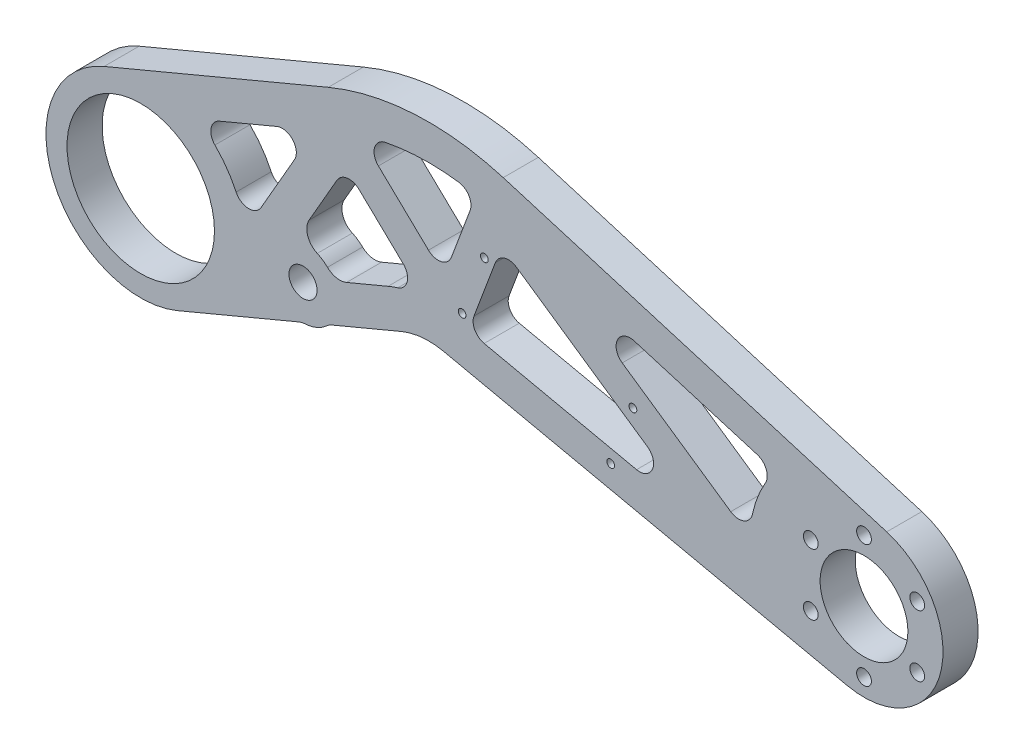
from build123d import *

# Parameters (mm, degrees)
SKETCH_1_R          = 21
SKETCH_1_R_2        = 12.5
EXTRUDE_1_DEPTH     = 10
EXTRUDE_3_DEPTH     = 10
CUT_EXTRUDE_1_DEPTH = 143.471558445
CUT_EXTRUDE_2_DEPTH = 143.471558445
FILLET_1_R          = 4
SKETCH_4_R          = 2.1
CUT_EXTRUDE_3_DEPTH = 143.471558445
SKETCH_5_R          = 4
CUT_EXTRUDE_4_DEPTH = 10
SKETCH_6_R          = 10
SKETCH_6_R_2        = 4
EXTRUDE_4_DEPTH     = 10
FILLET_2_R          = 5
SKETCH_7_R          = 1.1
CUT_EXTRUDE_5_DEPTH = 10


with BuildPart() as part:
    # 草图1 → 凸台-拉伸1 (new body)
    with BuildSketch(Plane.XY):
        with BuildLine():
            ThreePointArc((-102.410194175, 26.993557177), (-130, 0), (-102.410194175, -26.993557177))
            Line((-102.410194175, -26.993557177), (103.491504854, -22.494630981))
            ThreePointArc((103.491504854, -22.494630981), (125.5, 0), (103.491504854, 22.494630981))
            Line((103.491504854, 22.494630981), (-102.410194175, 26.993557177))
        make_face()
        with Locations((-103, 0)):
            Circle(SKETCH_1_R, mode=Mode.SUBTRACT)
        with Locations((103, 0)):
            Circle(SKETCH_1_R_2, mode=Mode.SUBTRACT)
    extrude(amount=EXTRUDE_1_DEPTH)

    # 草图2 → 凸台-拉伸3 (add)
    with BuildSketch(Plane(origin=(0, 0, 0), x_dir=(-1, 0, 0), z_dir=(0, 0, -1))):
        with BuildLine():
            Line((-103.491504854, 22.494630981), (-40.939702548, 23.861379985))
            ThreePointArc((-40.939702548, 23.861379985), (-23.289176704, 42.694903268), (-0.239881629, 54.312676651))
            Line((-0.239881629, 54.312676651), (-109.464232513, 21.551419861))
            ThreePointArc((-109.464232513, 21.551419861), (-106.509698333, 22.224581382), (-103.491504854, 22.494630981))
        make_face()
        with BuildLine():
            ThreePointArc((-0.239881629, 54.312676651), (-23.289176704, 42.694903268), (-40.939702548, 23.861379985))
            Line((-40.939702548, 23.861379985), (81.117648154, 26.528317728))
            ThreePointArc((81.117648154, 26.528317728), (67.102789284, 41.29360316), (49.592159014, 51.676654281))
            ThreePointArc((49.592159014, 51.676654281), (24.905271972, 57.326259535), (-0.239881629, 54.312676651))
        make_face()
        with BuildLine():
            ThreePointArc((49.592159014, 51.676654281), (67.102789284, 41.29360316), (81.117648154, 26.528317728))
            Line((81.117648154, 26.528317728), (102.410194175, 26.993557177))
            ThreePointArc((102.410194175, 26.993557177), (108.03630245, 26.526131599), (113.442225649, 24.898994428))
            Line((113.442225649, 24.898994428), (49.592159014, 51.676654281))
        make_face()
    extrude(amount=-EXTRUDE_3_DEPTH)

    # 草图2<4> → 切除-拉伸1 (cut, through all)
    with BuildSketch(Plane(origin=(0, 0, 0), x_dir=(-1, 0, 0), z_dir=(0, 0, -1))):
        with BuildLine():
            ThreePointArc((-98.226911662, -21.987897301), (-100.844267169, -22.396491153), (-103.491504854, -22.494630981))
            Line((-103.491504854, -22.494630981), (102.410194175, -26.993557177))
            ThreePointArc((102.410194175, -26.993557177), (97.385444996, -26.409785537), (92.557774351, -24.898994428))
            Line((92.557774351, -24.898994428), (28.707707717, 1.878665426))
            ThreePointArc((28.707707717, 1.878665426), (22.824400221, 3.34579716), (16.772215113, 2.97588088))
            Line((16.772215113, 2.97588088), (-98.226911662, -21.987897301))
        make_face()
    extrude(amount=-CUT_EXTRUDE_1_DEPTH, mode=Mode.SUBTRACT)

    # 草图3 → 切除-拉伸2 (cut, through all)
    with BuildSketch(Plane(origin=(0, 0, 0), x_dir=(-1, 0, 0), z_dir=(0, 0, -1))):
        with BuildLine():
            Line((-13.049437663, 40.030371792), (-77.856013804, 20.591987718))
            ThreePointArc((-77.856013804, 20.591987718), (-72.492161336, 11.2036503), (-70.505090985, 0.57522877))
            Line((-70.505090985, 0.57522877), (-13.049437663, 40.030371792))
        make_face()
        Polygon((0.198802543, 36.997209558), (-58.115751128, -3.047745505), (9.712361202, 11.67624413), align=None)
        with BuildLine():
            ThreePointArc((40.504408652, 44.381493291), (24.109384021, 47.353816747), (7.503136565, 45.988501819))
            Line((7.503136565, 45.988501819), (16.668465779, 21.594372082))
            Line((16.668465779, 21.594372082), (40.504408652, 44.381493291))
        make_face()
        with BuildLine():
            Line((44.567749988, 34.431544826), (22.556649299, 13.38896967))
            ThreePointArc((22.556649299, 13.38896967), (27.664879137, 12.677954881), (32.575198698, 11.100515214))
            Line((32.575198698, 11.100515214), (66.033457739, -2.931324174))
            Line((66.033457739, -2.931324174), (44.567749988, 34.431544826))
        make_face()
        with BuildLine():
            Line((86.779784403, 25.236969033), (53.321525362, 39.268808421))
            Line((53.321525362, 39.268808421), (73.33058295, 4.441361493))
            ThreePointArc((73.33058295, 4.441361493), (77.809150087, 16.291748852), (86.779784403, 25.236969033))
        make_face()
    extrude(amount=-CUT_EXTRUDE_2_DEPTH, mode=Mode.SUBTRACT)

    # 圆角1
    fillet_1_edges = [part.edges().sort_by_distance(p)[0] for p in [
        (-86.779784403, 25.236969033, 5),
        (-73.33058295, 4.441361493, 5),
        (-53.321525362, 39.268808421, 5),
        (-22.556649299, 13.38896967, 5),
        (-44.567749988, 34.431544826, 5),
        (-66.033457739, -2.931324174, 5),
        (70.505090985, 0.57522877, 5),
        (77.856013804, 20.591987718, 5),
        (13.049437663, 40.030371792, 5),
        (-40.504408652, 44.381493291, 5),
        (-16.668465779, 21.594372082, 5),
        (-7.503136565, 45.988501819, 5),
        (-0.198802543, 36.997209558, 5),
        (-9.712361202, 11.67624413, 5),
        (58.115751128, -3.047745505, 5),
    ]]
    fillet(fillet_1_edges, radius=FILLET_1_R)

    # 草图4 → 切除-拉伸3 (cut, through all)
    with BuildSketch(Plane.XY.offset(10)):
        with Locations((103, 17.5)):
            Circle(SKETCH_4_R)
        with Locations((118.155444566, 8.75)):
            Circle(SKETCH_4_R)
        with Locations((118.155444566, -8.75)):
            Circle(SKETCH_4_R)
        with Locations((103, -17.5)):
            Circle(SKETCH_4_R)
        with Locations((87.844555434, -8.75)):
            Circle(SKETCH_4_R)
        with Locations((87.844555434, 8.75)):
            Circle(SKETCH_4_R)
    extrude(amount=-CUT_EXTRUDE_3_DEPTH, mode=Mode.SUBTRACT)

    # 草图5 → 切除-拉伸4 (cut)
    with BuildSketch(Plane.XY.offset(10)):
        with Locations((-56.77893166, 0)):
            Circle(SKETCH_5_R)
    extrude(amount=-CUT_EXTRUDE_4_DEPTH, mode=Mode.SUBTRACT)

    # 草图6 → 凸台-拉伸4 (add)
    with BuildSketch(Plane.XY.offset(10)):
        with Locations((-56.77893166, 0)):
            Circle(SKETCH_6_R)
        with Locations((-56.77893166, 0)):
            Circle(SKETCH_6_R_2, mode=Mode.SUBTRACT)
    extrude(amount=-EXTRUDE_4_DEPTH)

    # 圆角2
    fillet_2_edges = [part.edges().sort_by_distance(p)[0] for p in [
        (-47.931305001, 4.660418705, 5),
        (-57.024626927, -9.996981236, 5),
        (-49.475805199, -6.831130499, 5),
        (-58.71258633, 9.811267992, 5),
    ]]
    fillet(fillet_2_edges, radius=FILLET_2_R)

    # 草图7 → 切除-拉伸5 (cut)
    with BuildSketch(Plane.XY.offset(10)):
        with Locations((-5.129756774, 31.838429538)):
            Circle(SKETCH_7_R)
        with Locations((-11.460593594, 14.988488732)):
            Circle(SKETCH_7_R)
        with Locations((37.182316805, 15.940994857)):
            Circle(SKETCH_7_R)
        with Locations((30.851479985, -0.908945949)):
            Circle(SKETCH_7_R)
    extrude(amount=-CUT_EXTRUDE_5_DEPTH, mode=Mode.SUBTRACT)


solid = part.part
